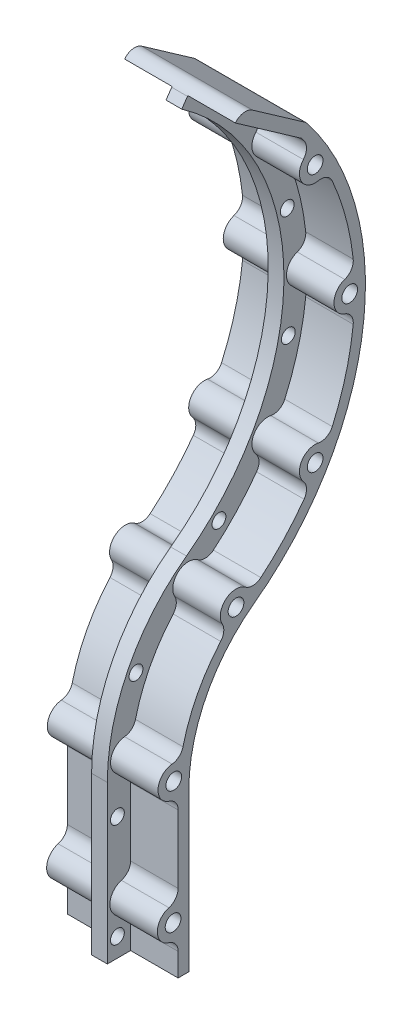
from build123d import *

# Parameters (mm, degrees)
SKETCH_3_R         = 1.0999999999999992
SKETCH_3_R_2       = 1.100000000000007
SKETCH_3_R_3       = 1.0999999999999983
EXTRUDE_1_DEPTH    = 1.25
EXTRUDE_2_DEPTH    = 8.8
HOLE_WIZARD_M3_1_D = 2.5
FILLET_R2_1_R      = 2


with BuildPart() as part:
    # 草图3 → 凸台-拉伸1 (new, symmetric)
    with BuildSketch(Plane(origin=(0, 0, 0), x_dir=(0, 0, -1), z_dir=(1, 0, 0))):
        with BuildLine():
            Line((19.5, -3.12e-15), (19.500000000000004, -25.00000000000001))
            Line((19.500000000000004, -25.00000000000001), (14.100000000000005, -25.00000000000001))
            Line((14.100000000000005, -25.00000000000001), (14.100000000000001, 0))
            ThreePointArc((14.100000000000001, 0), (17.421526991333195, 13.936923136411288), (26.672027605840533, 24.877608967079777))
            ThreePointArc((26.672027605840533, 24.877608967079777), (42.17069683857236, 56.010769758457506), (25.926721927337365, 86.76163524108378))
            Line((25.926721927337365, 86.76163524108378), (27.985996640623934, 89.70258431819843))
            Line((27.985996640623934, 89.70258431819843), (38.157154957885716, 82.58066259212733))
            ThreePointArc((38.157154957885716, 82.58066259212733), (47.19107481579925, 49.796834454639864), (29.874974237829562, 20.530065652444478))
            ThreePointArc((29.874974237829562, 20.530065652444478), (22.241065963721567, 11.501344335873394), (19.5, -3.12e-15))
        make_face()
        with Locations((15.700000000000003, -22.000000000000014)):
            Circle(SKETCH_3_R, mode=Mode.SUBTRACT)
        with Locations((15.700000000000003, -5.5000000000000115)):
            Circle(SKETCH_3_R, mode=Mode.SUBTRACT)
        with Locations((18.656131284605202, 12.825388146408793)):
            Circle(SKETCH_3_R, mode=Mode.SUBTRACT)
        with Locations((42.69345970236235, 64.74898535672597)):
            Circle(SKETCH_3_R_2, mode=Mode.SUBTRACT)
        with Locations((31.841454389394453, 27.178918703364943)):
            Circle(SKETCH_3_R, mode=Mode.SUBTRACT)
        with Locations((42.86604311676676, 47.112423881836435)):
            Circle(SKETCH_3_R_3, mode=Mode.SUBTRACT)
    extrude(amount=EXTRUDE_1_DEPTH, both=True)

    # 草图4 → 凸台-拉伸2 (add, symmetric)
    with BuildSketch(Plane(origin=(0, 0, 0), x_dir=(0, 0, -1), z_dir=(1, 0, 0))):
        with BuildLine():
            Line((19.500000000000004, 3.12e-15), (19.500000000000004, -25.00000000000001))
            Line((19.500000000000004, -25.00000000000001), (17.800000000000004, -25.00000000000001))
            Line((17.800000000000004, -25.00000000000001), (17.800000000000004, -19.368543856465415))
            ThreePointArc((17.800000000000004, -19.368543856465415), (14.5, -17.00000000000001), (17.800000000000004, -14.63145614353461))
            Line((17.800000000000004, -14.63145614353461), (17.800000000000004, 0.03846051745544626))
            ThreePointArc((17.800000000000004, 0.03846051745544626), (14.616062942086879, 2.658264256715171), (18.206575944742145, 4.685341758626529))
            ThreePointArc((18.206575944742145, 4.685341758626529), (20.873305337552384, 12.559562279992942), (25.793916032971335, 19.2604864593666))
            ThreePointArc((25.793916032971335, 19.2604864593666), (25.390331087301867, 23.36044674604562), (29.363264344403504, 22.270329093985996))
            ThreePointArc((29.363264344403504, 22.270329093985996), (34.63201747726785, 27.031519027261), (39.01879216923118, 32.61586294196908))
            ThreePointArc((39.01879216923118, 32.61586294196908), (37.41543774806319, 36.301942353673255), (41.409353369549805, 36.75643639952374))
            ThreePointArc((41.409353369549805, 36.75643639952374), (44.44915924124539, 44.73330626838789), (45.805045068215996, 53.16138115335468))
            ThreePointArc((45.805045068215996, 53.16138115335468), (42.57345970236232, 55.5519423536733), (45.805045068215996, 57.94250355399191))
            ThreePointArc((45.805045068215996, 57.94250355399191), (44.44915924124538, 66.3705784389587), (41.409353369549805, 74.34744830782286))
            ThreePointArc((41.409353369549805, 74.34744830782286), (37.41543774806319, 74.80194235367335), (39.01879216923118, 78.48802176537752))
            ThreePointArc((39.01879216923118, 78.48802176537752), (38.22185794799814, 79.65851608901482), (37.38573446811181, 80.80134531554968))
            Line((37.38573446811181, 80.80134531554968), (26.896201411556945, 88.14619543404935))
            Line((26.896201411556945, 88.14619543404935), (27.985996640623934, 89.70258431819843))
            Line((27.985996640623934, 89.70258431819843), (38.1571549578857, 82.58066259212734))
            ThreePointArc((38.1571549578857, 82.58066259212734), (47.19107481579925, 49.79683445463986), (29.874974237829548, 20.530065652444467))
            ThreePointArc((29.874974237829548, 20.530065652444467), (22.24106596372156, 11.501344335873386), (19.500000000000004, 3.12e-15))
        make_face()
    extrude(amount=EXTRUDE_2_DEPTH, both=True)

    # M3 螺纹孔1 (through all)
    with Locations(Plane(origin=(8.8, 0, 0), x_dir=(0, 0, -1), z_dir=(1, 0, 0))):
        with Locations((39.580501258, 76.051942354), (45.073459702, 55.551942354), (39.580501258, 35.051942354), (27.001946929, 21.449244407), (17.106548453, 2.440360797), (17, -17)):
            Hole(HOLE_WIZARD_M3_1_D / 2)

    # R2 圆角1
    fillet_r2_1_edges = [part.edges().sort_by_distance(p)[0] for p in [
        (0, 82.58066259212734, -38.15715495788571),
        (0, 89.70258431819843, -27.985996640623934),
        (5.025, -19.368543856465415, -17.800000000000004),
        (-5.025, -19.368543856465415, -17.800000000000004),
        (-5.025, -14.63145614353461, -17.800000000000004),
        (5.025, -14.63145614353461, -17.800000000000004),
        (5.025, 0.03846051745544712, -17.800000000000004),
        (-5.025, 0.03846051745544712, -17.800000000000004),
        (-5.025, 4.68534175862653, -18.20657594474214),
        (5.025, 4.68534175862653, -18.20657594474214),
        (-5.025, 19.260486459366604, -25.79391603297133),
        (5.025, 19.260486459366604, -25.79391603297133),
        (-5.025, 22.270329093985993, -29.363264344403504),
        (5.025, 22.270329093985993, -29.363264344403504),
        (-5.025, 32.61586294196907, -39.01879216923119),
        (5.025, 32.61586294196907, -39.01879216923119),
        (-5.025, 36.756436399523736, -41.409353369549805),
        (5.025, 36.756436399523736, -41.409353369549805),
        (-5.025, 53.16138115335468, -45.805045068216),
        (5.025, 53.16138115335468, -45.805045068216),
        (5.025, 57.94250355399191, -45.80504506821599),
        (-5.025, 57.94250355399191, -45.80504506821599),
        (5.025, 74.34744830782286, -41.409353369549805),
        (-5.025, 74.34744830782286, -41.409353369549805),
        (-5.025, 78.48802176537752, -39.01879216923119),
        (5.025, 78.48802176537752, -39.01879216923119),
    ]]
    fillet(fillet_r2_1_edges, radius=FILLET_R2_1_R)


solid = part.part
